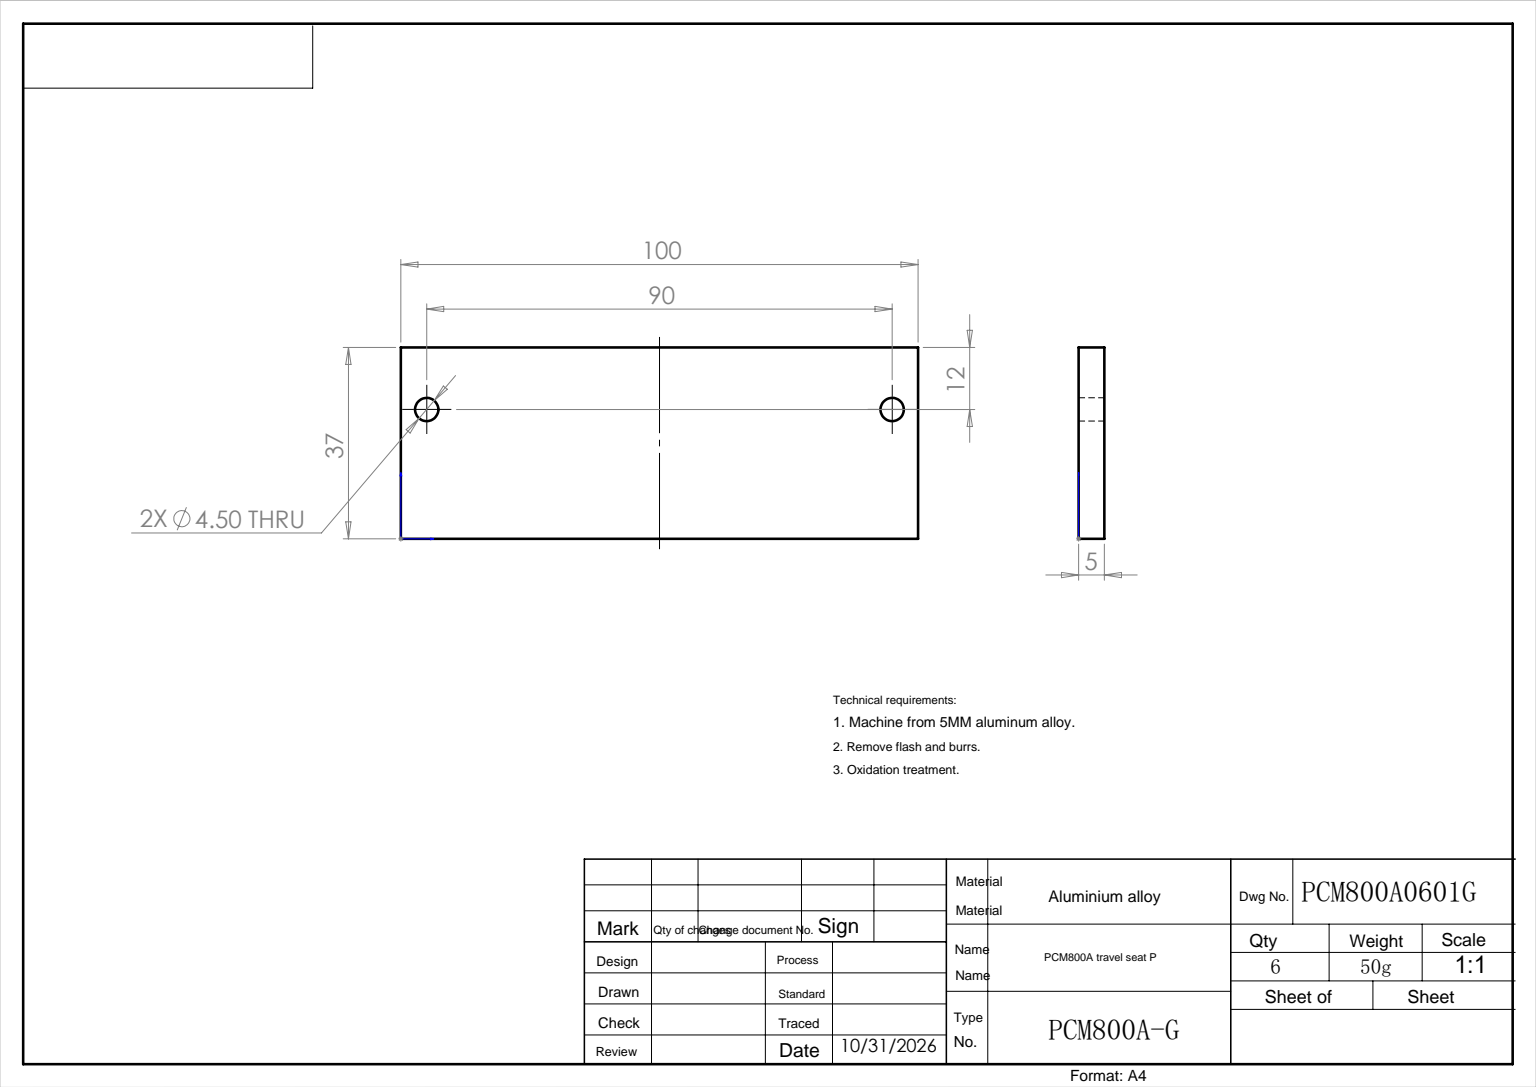
from build123d import *

# Parameters (mm, degrees)
SKETCH_1_W          = 100
SKETCH_1_H          = 37
EXTRUDE_1_DEPTH     = 5
SKETCH_2_R          = 2.25
CUT_EXTRUDE_1_DEPTH = 5


with BuildPart() as part:
    # 草图1 → 凸台-拉伸1 (new body)
    with BuildSketch(Plane.XY):
        with Locations((50, 18.5)):
            Rectangle(SKETCH_1_W, SKETCH_1_H)
    extrude(amount=EXTRUDE_1_DEPTH)

    # 草图2 → 切除-拉伸1 (cut)
    with BuildSketch(Plane.XY.offset(5)):
        with Locations((5, 25)):
            Circle(SKETCH_2_R)
        with Locations((95, 25)):
            Circle(SKETCH_2_R)
    extrude(amount=-CUT_EXTRUDE_1_DEPTH, mode=Mode.SUBTRACT)


solid = part.part
